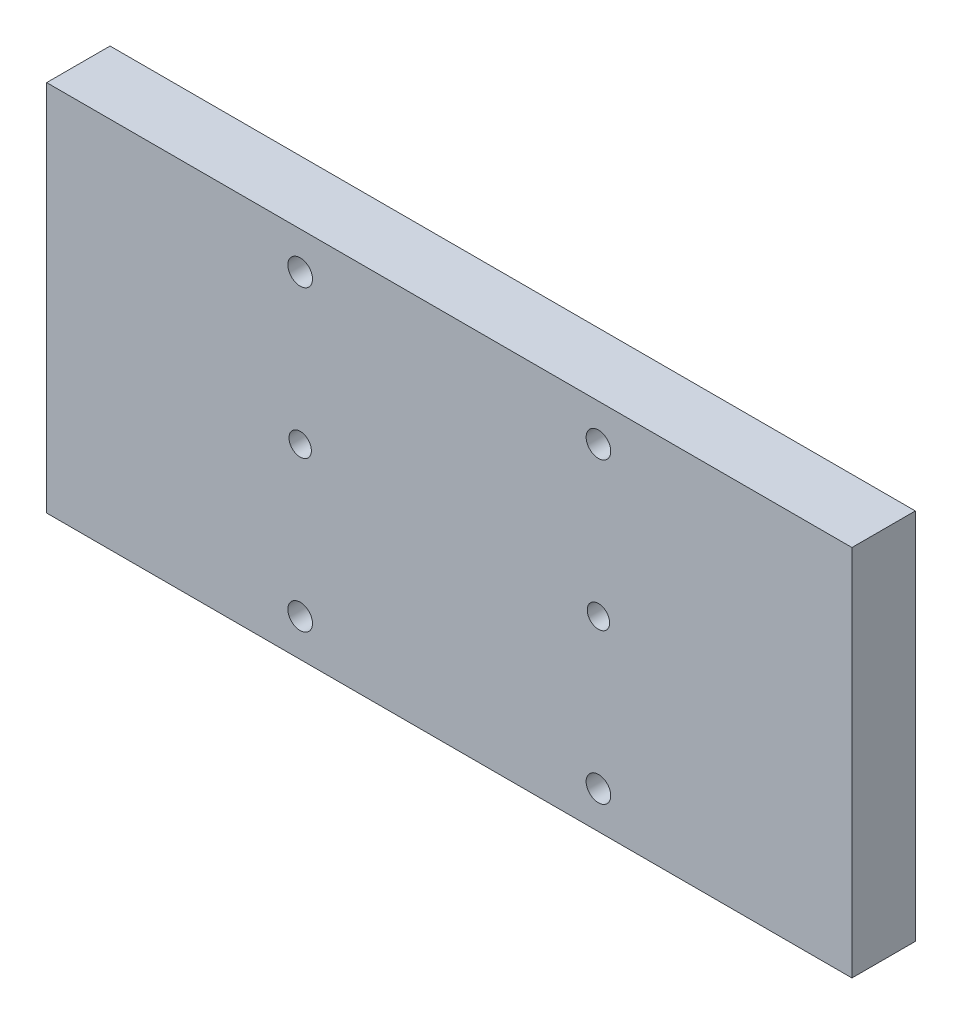
SolidWorks part; units mm, degrees
ref_plane "Front Plane" through (0, 0, 0) normal (0, 0, 1) x (1, 0, 0)
ref_plane "Top Plane" through (0, 0, 0) normal (0, 1, 0) x (1, 0, 0)
ref_plane "Right Plane" through (0, 0, 0) normal (1, 0, 0) x (0, 0, -1)
ref_plane "Plane1" through (0, 0, 0) normal (0, 0, -1) x (-1, 0, 0)
sketch "Sketch1" plane through (0, 0, 0) normal (0, 0, -1) x (-1, 0, 0)
  line L0 (108, 50) -> (-108, 50)
  line L1 (-108, 50) -> (-108, -50)
  line L2 (-108, -50) -> (108, -50)
  line L3 (108, -50) -> (108, 50)
extrude "Boss-Extrude1" add sketch "Sketch1" against normal blind 17
hole_wizard "Ø6.0 (6) Diameter Hole1" positions "Sketch7" profile "Sketch6" hole size "Ø6.0" standard "ANSI Metric"
sketch "Sketch7" plane through (0, 0, 0) normal (0, 0, -1) x (-1, 0, 0)
  point P0 (-40, 0)
  point P1 (40, 0)
sketch "Sketch6" plane through (40, 0, 0) normal (1, 0, 0) x (0, 1, 0)
  line L0 (0, 0) -> (0, 17)
  line L1 (0, 17) -> (3, 17)
  line L2 (3, 17) -> (3, 0)
  line L5 (3, 0) -> (0, 0)
  line L11 (0, -6.35) -> (0, 107.95) construction
  dimension "通孔孔直径" = 6
  dimension "通孔孔深度" = 17
hole_wizard "CBORE for M6 Hex Head Bolt1" positions "Sketch9" profile "Sketch8" counterbore size "M6" standard "ANSI Metric"
sketch "Sketch9" plane through (0, 0, 0) normal (0, 0, -1) x (-1, 0, 0)
  point P0 (40, 40)
  point P1 (40, -40)
  point P2 (-40, -40)
  point P3 (-40, 40)
sketch "Sketch8" plane through (-40, 40, 0) normal (1, 0, 0) x (0, 1, 0)
  line L0 (0, 0) -> (0, 17)
  line L1 (0, 17) -> (3.3, 17)
  line L3 (3.3, 17) -> (3.3, 6.8)
  line L4 (3.3, 6.8) -> (5.5, 6.8)
  line L5 (5.5, 6.8) -> (5.5, 0)
  line L7 (5.5, 0) -> (0, 0)
  line L11 (0, -6.35) -> (0, 107.95) construction
  dimension "通孔孔直径" = 6.6
  dimension "通孔孔深度" = 17
  dimension "柱形沉头孔直径" = 11
  dimension "柱形沉头孔深度" = 6.8
